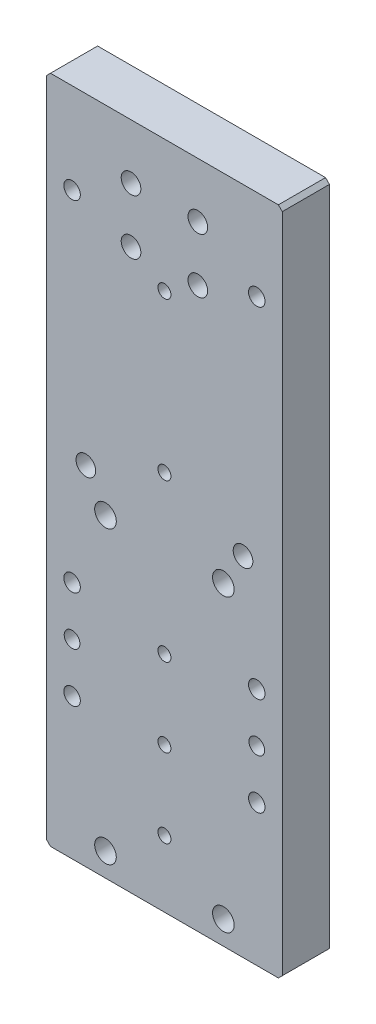
from build123d import *

# Parameters (mm, degrees)
SKETCH1_W                                           = 60
SKETCH1_H                                           = 170.4
BOSS_EXTRUDE1_DEPTH                                 = 6
CBORE_FOR_M5_HEX_SOCKET_HEAD_CAP_SCREW1_D           = 5.5
CBORE_FOR_M5_HEX_SOCKET_HEAD_CAP_SCREW1_CBORE_D     = 10
CBORE_FOR_M5_HEX_SOCKET_HEAD_CAP_SCREW1_CBORE_DEPTH = 5.4
BLIND_PIN_HOLE0_D                                   = 5
M4_TAPPED_HOLE1_D                                   = 3.3
SKETCH11_R                                          = 3.5
CUT_EXTRUDE1_DEPTH                                  = 2
M6_TAPPED_HOLE1_D                                   = 5
M6_TAPPED_HOLE1_DEPTH                               = 17
M6_TAPPED_HOLE1_TIP                                 = 1.502151548
CHAMFER1_SIZE                                       = 1
BLIND_PIN_HOLE1_D                                   = 4
M5_TAPPED_HOLE1_D                                   = 4.2


with BuildPart() as part:
    # Sketch1 → Boss-Extrude1 (new, symmetric)
    with BuildSketch(Plane.XY):
        Rectangle(SKETCH1_W, SKETCH1_H)
    extrude(amount=BOSS_EXTRUDE1_DEPTH, both=True)

    # CBORE for M5 Hex Socket Head Cap Screw1 (through all)
    with Locations(Plane(origin=(0, 0, -6), x_dir=(-1, 0, 0), z_dir=(0, 0, -1))):
        with Locations((15, -5.2), (-15, -5.2), (15, -79.2), (-15, -79.2)):
            CounterBoreHole(CBORE_FOR_M5_HEX_SOCKET_HEAD_CAP_SCREW1_D / 2, CBORE_FOR_M5_HEX_SOCKET_HEAD_CAP_SCREW1_CBORE_D / 2, CBORE_FOR_M5_HEX_SOCKET_HEAD_CAP_SCREW1_CBORE_DEPTH)

    # Blind pin hole0 (through all)
    with Locations(Plane.XY.offset(6)):
        with Locations((20, 3.3), (-20, 3.3)):
            Hole(BLIND_PIN_HOLE0_D / 2)

    # M4 Tapped Hole1 (through all)
    with Locations(Plane(origin=(0, 0, -6), x_dir=(-1, 0, 0), z_dir=(0, 0, -1))):
        with Locations((0, 11.7), (0, -28.3), (0, -48.3), (0, -68.3), (0, 51.7)):
            Hole(M4_TAPPED_HOLE1_D / 2)

    # Sketch11 → Cut-Extrude1 (cut)
    with BuildSketch(Plane(origin=(0, 0, -6), x_dir=(-1, 0, 0), z_dir=(0, 0, -1))):
        with Locations((0, 51.7)):
            Circle(SKETCH11_R)
        with Locations((0, -68.3)):
            Circle(SKETCH11_R)
    extrude(amount=-CUT_EXTRUDE1_DEPTH, mode=Mode.SUBTRACT)

    # M6 Tapped Hole1
    with Locations(Plane.XY.offset(6)):
        with Locations((8.5, 57.2), (-8.5, 57.2), (8.5, 71.2), (-8.5, 71.2)):
            Hole(M6_TAPPED_HOLE1_D / 2, depth=M6_TAPPED_HOLE1_DEPTH)
            with Locations((0, 0, -(M6_TAPPED_HOLE1_DEPTH + M6_TAPPED_HOLE1_TIP / 2))):  # 118° drill point
                Cone(0, M6_TAPPED_HOLE1_D / 2, M6_TAPPED_HOLE1_TIP, mode=Mode.SUBTRACT)

    # Chamfer1
    chamfer1_edges = [part.edges().sort_by_distance(p)[0] for p in [
        (30, -85.2, 0),
        (-30, -85.2, 0),
        (-30, 85.2, 0),
        (30, 85.2, 0),
    ]]
    chamfer(chamfer1_edges, length=CHAMFER1_SIZE)

    # Blind pin hole1 (through all)
    with Locations(Plane(origin=(0, 0, -6), x_dir=(-1, 0, 0), z_dir=(0, 0, -1))):
        with Locations((23.5, -36.8), (-23.5, -36.8)):
            Hole(BLIND_PIN_HOLE1_D / 2)

    # M5 Tapped Hole1 (through all)
    with Locations(Plane(origin=(0, 0, -6), x_dir=(-1, 0, 0), z_dir=(0, 0, -1))):
        with Locations((23.5, 62.2), (-23.5, -24.3), (-23.5, -49.3), (23.5, -49.3), (23.5, -24.3), (-23.5, 62.2)):
            Hole(M5_TAPPED_HOLE1_D / 2)


solid = part.part
